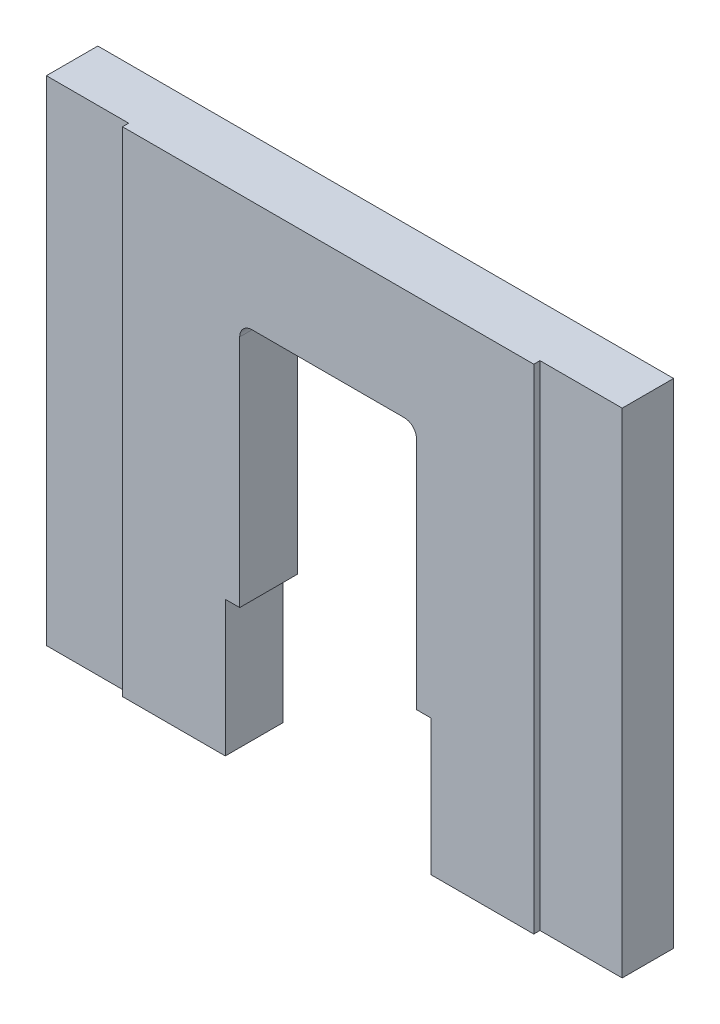
SolidWorks part; units mm, degrees
ref_plane "前视基准面" through (0, 0, 0) normal (0, 0, 1) x (1, 0, 0)
ref_plane "上视基准面" through (0, 0, 0) normal (0, 1, 0) x (1, 0, 0)
ref_plane "右视基准面" through (0, 0, 0) normal (1, 0, 0) x (0, 0, -1)
sketch "草图1" plane through (0, 0, 0) normal (0, 0, 1) x (1, 0, 0)
  line L1 (-70, -60) -> (70, -60)
  line L2 (-70, -60) -> (-70, 60)
  line L3 (-70, 60) -> (70, 60)
  line L4 (70, -60) -> (70, 60)
  line L5 (-70, -60) -> (70, 60) construction
  line L6 (-70, 60) -> (70, -60) construction
  point P0 (0, 0)
  dimension "D1" = 140
  dimension "D2" = 120
extrude "凸台-拉伸1" add sketch "草图1" along normal blind 14
sketch "草图2" plane through (0, 0, 14) normal (0, 0, 1) x (1, 0, 0)
  line L0 (-70, -60) -> (70, -60) construction
  line L1 (-70, 60) -> (-50, 60)
  line L2 (-70, 60) -> (-70, -60)
  line L3 (-70, -60) -> (-50, -60)
  line L4 (-50, 60) -> (-50, -60)
  line L6 (70, 60) -> (50, 60)
  line L7 (70, 60) -> (70, -60)
  line L8 (70, -60) -> (50, -60)
  line L9 (50, 60) -> (50, -60)
  dimension "D1" = 20
extrude "切除-拉伸1" cut sketch "草图2" against normal blind 1.5
sketch "草图3" plane through (0, 0, 14) normal (0, 0, 1) x (1, 0, 0)
  line L0 (25, -60) -> (25, -27)
  line L1 (-50, -60) -> (50, -60) construction
  line L2 (25, -27) -> (-25, -27)
  line L3 (-25, -27) -> (-25, -60)
  line L4 (-25, -60) -> (25, -60)
  line L5 (-50, -60) -> (-50, 60) construction
  line L6 (50, 60) -> (50, -60) construction
  line L7 (50, 60) -> (-50, 60) construction
extrude "切除-拉伸2" cut sketch "草图3" against normal up to next
sketch "草图4" plane through (0, 0, 0) normal (0, 0, -1) x (-1, 0, 0)
  line L0 (21.5, -27) -> (21.5, 33)
  line L1 (-25, -27) -> (25, -27) construction
  line L2 (21.5, 33) -> (-21.5, 33)
  line L3 (-21.5, 33) -> (-21.5, -27)
  line L4 (-21.5, -27) -> (21.5, -27)
  line L5 (0, 33) -> (0, 0) construction
  dimension "D1" = 60
  dimension "D2" = 43
extrude "切除-拉伸3" cut sketch "草图4" against normal up to next and the other way through all
fillet "圆角1" radius 3 2 edges at (21.5, 33, 7) (-21.5, 33, 7)
equation "\"D2@草图3\"=\"D1@草图3\""
